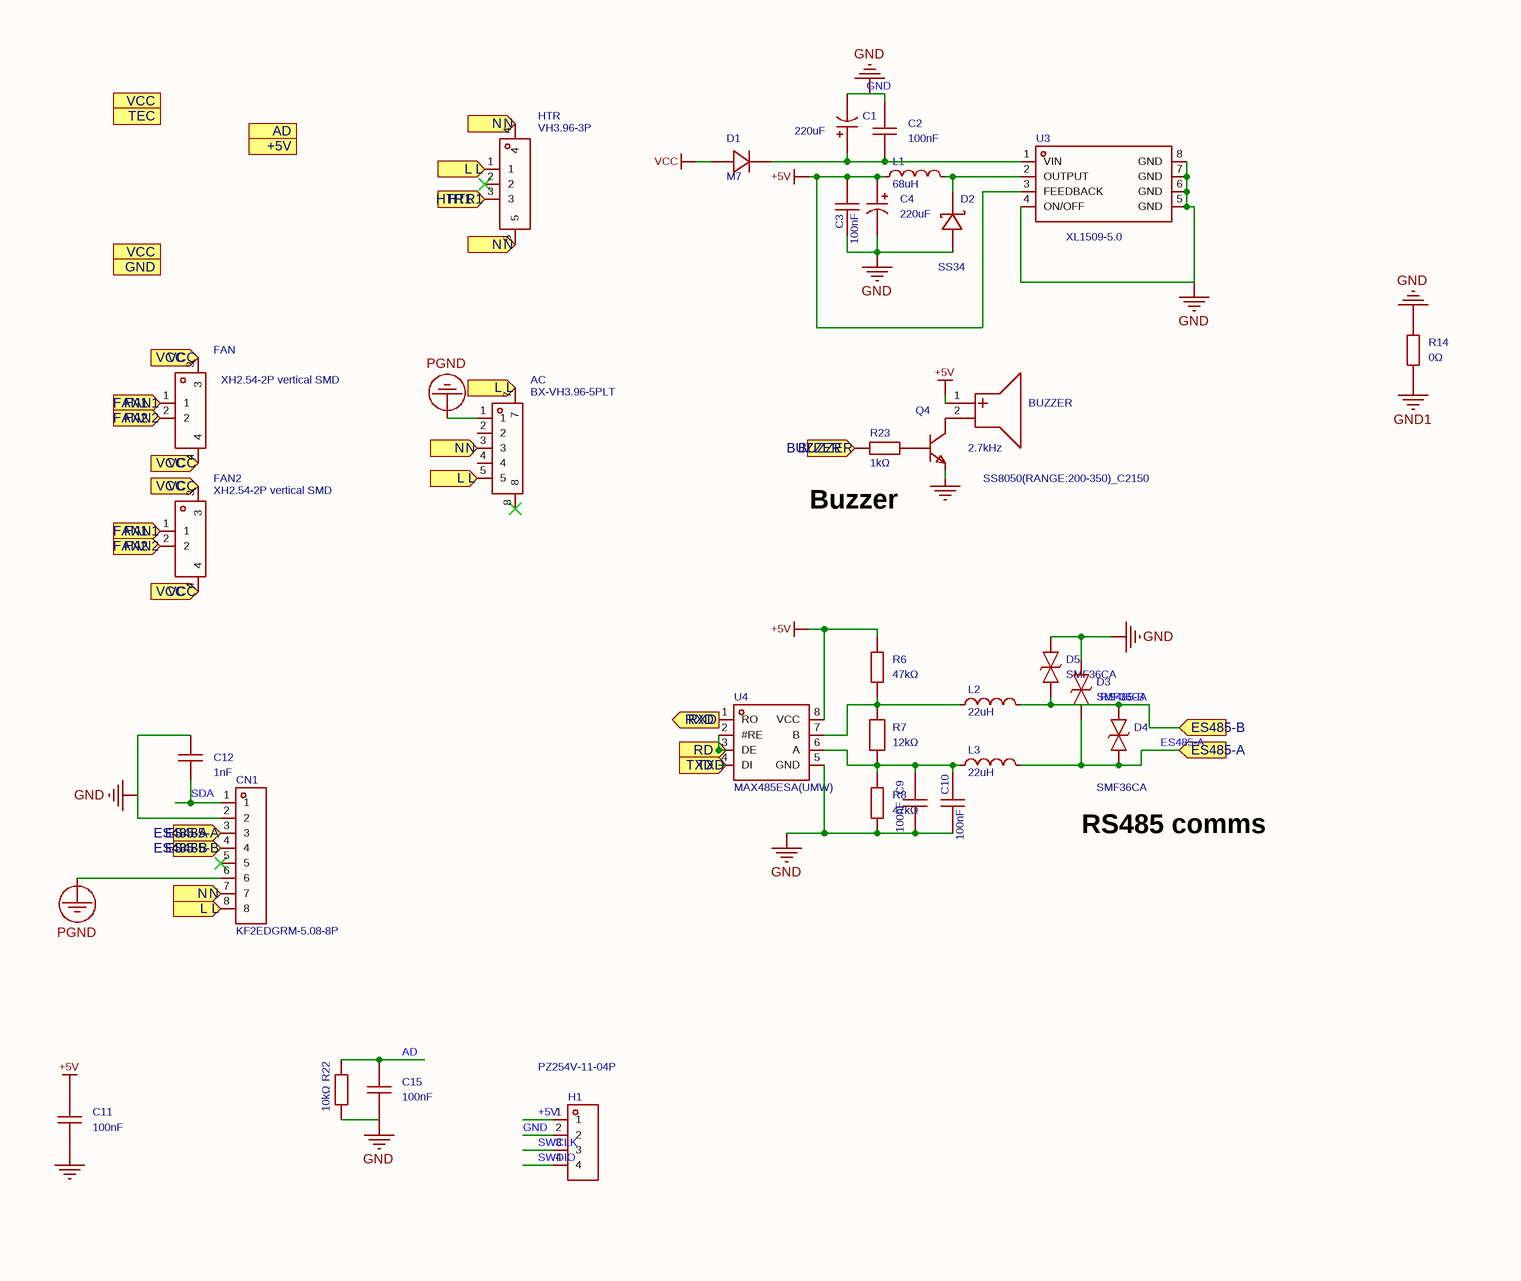
[diagram p0: MISC84275-2.SchDoc, left]
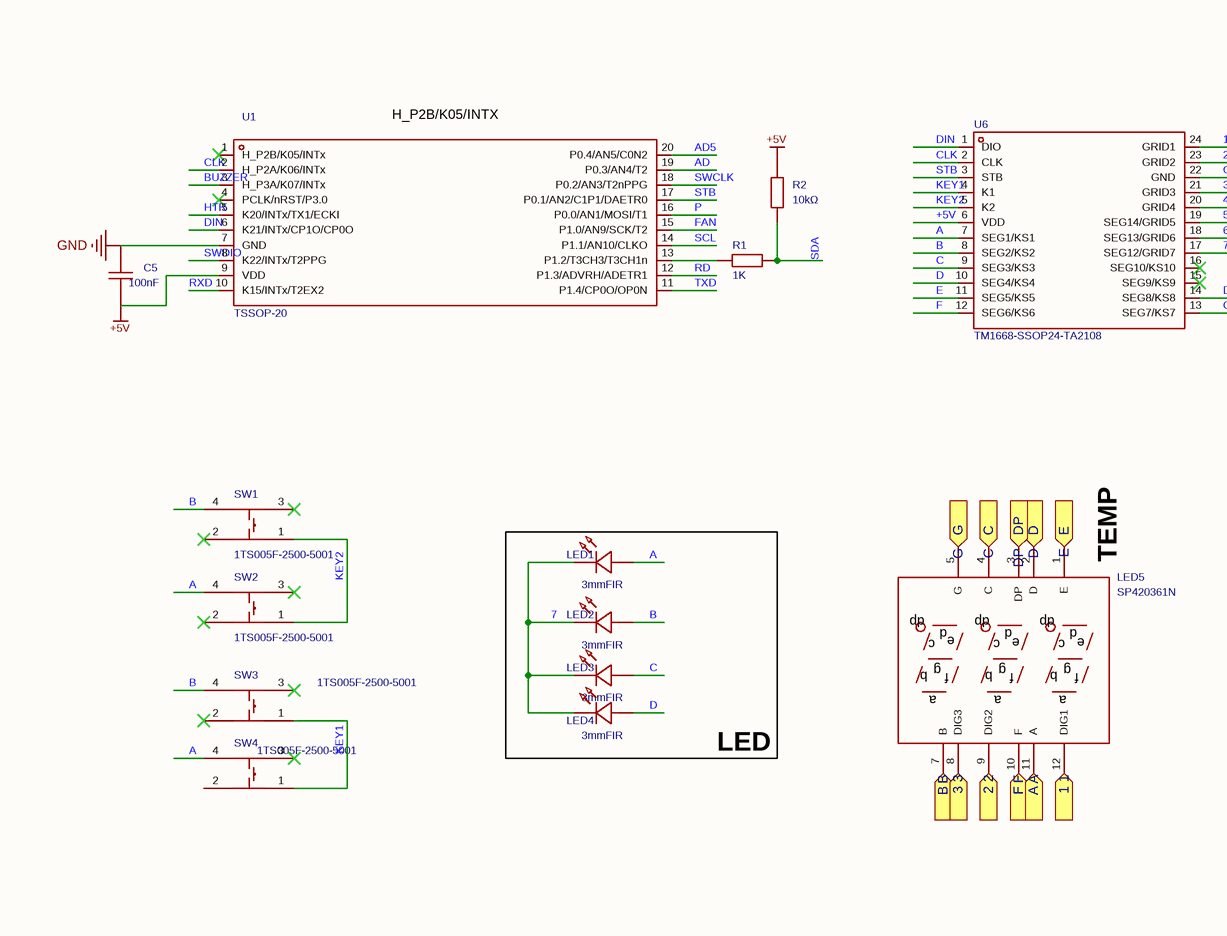
[diagram p1: MISC84275-2.SchDoc, middle]
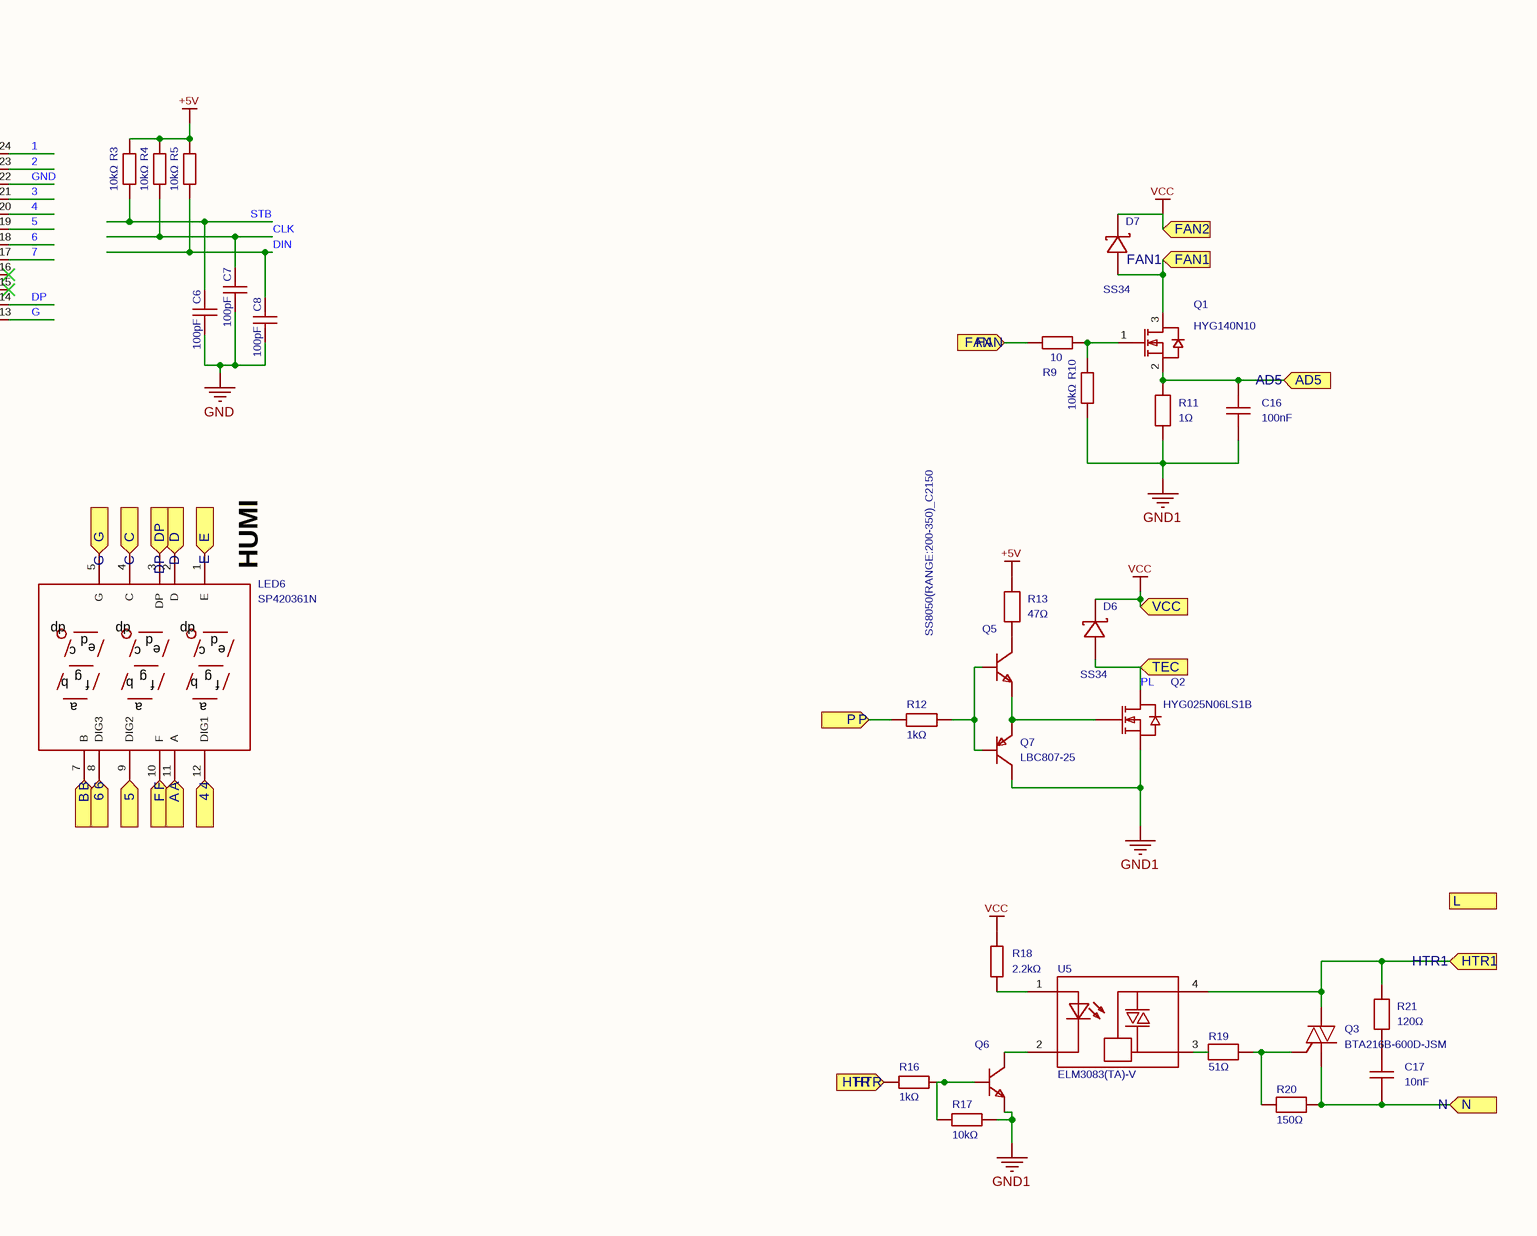
[diagram p2: MISC84275-2.SchDoc, right]
# Altium project MISC84275.PrjPcb (part 1 of 2)
1 sheet, 76 parts. Net scope: flat (ports and power ports of the same name join across sheets).
Board file: MISC84275.PcbDoc

## Sheet MISC84275-2.SchDoc
size 297 x 209 mm; Symbol: Drawing-Symbol_A4; Company: JLCEDA; Version: V1.0; Page Size: A4; @Project Name: Dehumidifier; @Page Count: 2; @Update Date: 2025-12-25; @Create Date: 2025-12-25; @Schematic Name: EDA-2150; @Page No: 1; @Page Name: P1; @Create Time: 08:36:43; @Update Time: 17:27:34; Border: 1; Width: 1170; Height: 825; Region Start: 1; X Region Count: 6; Y Region Count: 4; Blade Width: 10; Title Block Position: 3; @Board Name: EDA-2150; Device: Drawing-Symbol_A4

### Parts
AC  BX-VH3.96-5PLT  [CONN-SMD_5P-P3.96_BX-VH3.96-5PLT]
BUZZER  2.7kHz  [BUZ-SMD_L9.6-W9.6-LS10.0-R]
C1  220uF  [CAP-SMD_BD6.3-L6.6-W6.6-FD]
C2  100nF  [C0805]
C3  100nF  [C0805]
C4  220uF  [CAP-SMD_BD6.3-L6.6-W6.6-FD]
C5  100nF  [C0805]
C6  100pF  [C0805]
C7  100pF  [C0805]
C8  100pF  [C0805]
C9  100nF  [C0805]
C10  100nF  [C0805]
C11  100nF  [C0805]
C12  1nF  [C0805]
C15  100nF  [C0805]
C16  100nF  [C0805]
C17  10nF  [C1210]
CN1  KF2EDGRM-5.08-8P  [CONN-TH_8P-P5.08_KF2EDGRM-5.08-8P]
D1  M7  [SMA_L4.4-W2.8-LS5.4-RD]
D2  SS34  [SMA_L4.3-W2.6-LS5.2-RD]
D3  SMF36CA  [SOD-123_L2.7-W1.8-LS3.7-BI]
D4  SMF36CA  [SOD-123_L2.7-W1.8-LS3.7-BI]
D5  SMF36CA  [SOD-123_L2.7-W1.8-LS3.7-BI]
D6  SS34  [SMA_L4.3-W2.6-LS5.2-RD]
D7  SS34  [SMA_L4.3-W2.6-LS5.2-RD]
FAN  XH2.54-2P vertical SMD  [CONN-SMD_2P_A2501WV-S]
FAN2  XH2.54-2P vertical SMD  [CONN-SMD_2P_A2501WV-S]
H1  PZ254V-11-04P  [HDR-TH_4P-P2.54-V-M]
HTR  VH3.96-3P  [CONN-SMD_3P-P3.96_HCTL_HC-VH-3ALT]
L1  68uH  [IND-SMD_L7.1-W6.6_H5.0]
L2  22uH  [L1206]
L3  22uH  [L1206]
LED1  3mmFIR  [LED-TH_BD3.0-P2.54-FD]
LED2  3mmFIR  [LED-TH_BD3.0-P2.54-FD]
LED3  3mmFIR  [LED-TH_BD3.0-P2.54-FD]
LED4  3mmFIR  [LED-TH_BD3.0-P2.54-FD]
LED5  SP420361N  [LED-SEG-TH_SP420361N]
LED6  SP420361N  [LED-SEG-TH_SP420361N]
Q1  HYG140N10  [TO-252-3_L6.6-W6.1-P4.58-LS10.1-BR]
Q2  HYG025N06LS1B  [TO-263-2_L10.2-W8.7-P5.08-LS15.1-BR]
Q3  BTA216B-600D-JSM  [TO-263-3_L10.2-W9.2-P5.08-LS15.4-BR]
Q4  SS8050(RANGE:200-350)  [SOT-23-3_L2.9-W1.3-P1.90-LS2.4-BR]  (value not drawn)
Q5  SS8050(RANGE:200-350)  [SOT-23-3_L2.9-W1.3-P1.90-LS2.4-BR]  (value not drawn)
Q6  SS8050(RANGE:200-350)  [SOT-23-3_L2.9-W1.3-P1.90-LS2.4-BR]  (value not drawn)
Q7  LBC807-25  [SOT-23-3_L2.9-W1.6-P1.90-LS2.8-BR]
R1  1K  [R0805]
R2  10kΩ  [R0805]
R3  10kΩ  [R0805]
R4  10kΩ  [R0805]
R5  10kΩ  [R0805]
R6  47kΩ  [R0805]
R7  12kΩ  [R0805]
R8  47kΩ  [R0805]
R9  10  [R0805]
R10  10kΩ  [R0805]
R11  1Ω  [R1206]
R12  1kΩ  [R0805]
R13  47Ω  [R0805]
R14  0Ω  [R0603]
R16  1kΩ  [R0805]
R17  10kΩ  [R0805]
R18  2.2kΩ  [R0805]
R19  51Ω  [R0204]
R20  150Ω  [R0204]
R21  120Ω  [R0204]
R22  10kΩ  [R0805]
R23  1kΩ  [R0805]
SW1  1TS005F-2500-5001  [SW-SMD_4P-L6.0-W6.0-P4.50-LS9.0-H2.5]
SW2  1TS005F-2500-5001  [SW-SMD_4P-L6.0-W6.0-P4.50-LS9.0-H2.5]
SW3  1TS005F-2500-5001  [SW-SMD_4P-L6.0-W6.0-P4.50-LS9.0-H2.5]
SW4  1TS005F-2500-5001  [SW-SMD_4P-L6.0-W6.0-P4.50-LS9.0-H2.5]
U1  TSSOP-20  [TSSOP-20_L6.5-W4.4-P0.65-LS6.4-BL]
U3  XL1509-5.0  [SOIC-8_L4.9-W3.9-P1.27-LS6.0-TR]
U4  MAX485ESA(UMW)  [SOP-8_L5.0-W4.0-P1.27-LS6.0-BL]
U5  ELM3083(TA)-V  [SOP-4_L4.4-W4.0-P2.54-LS7.0-TL]
U6  TM1668-SSOP24-TA2108  [SSOP-24_L8.1-W5.3-P0.65-LS7.8-BL]

### Blocks framed on the sheet
LED: LED1-LED4

### Ports
1 (in), 2 (in), 3 (in), 4 (in), 5 (in), 6 (in), +5V (in), A (in), AD5 (in), AD (in), B (in), BUZZER (in), C (in), D (in), DP (in), E (in), ES485-A (in), ES485-B (in), F (in), FAN1 (in), FAN2 (in), FAN (in), G (in), GND (in), HTR1 (in), HTR (in), L (in), N (in), P (in), RD (in), RXD (out), TEC (in), TXD (in), VCC (in)

### Nets
+5V: BUZZER.1(+) C3.2 C4.1 C5.1 C11.2 H1.1 L1.1 R2.2 R3.2 R4.2 R5.2 R6.2 R13.2 U1.9(VDD) U3.3(FEEDBACK) U4.8(VCC) U6.6(VDD)
VCC: D1.2(A) D6.1(K) D7.1(K) FAN.2 FAN.3 FAN.4 FAN2.2 FAN2.3 FAN2.4 R18.2 ; port VCC, port FAN2  [also labelled FAN2]
GND: C1.2 C2.2 C3.1 C4.2 C5.2 C6.1 C7.1 C8.1 C9.1 C10.1 C11.1 C12.2 C15.1 CN1.2 D2.2(A) D3.2 D5.2 H1.2 Q4.2(E) R8.1 R14.2 R22.1 U1.7(GND) U3.4(ON/OFF) U3.5(GND) U3.6(GND) U3.7(GND) U3.8(GND) U4.5(GND) U6.22(GND)
GND1: C16.1 Q2.3(S) Q6.2(E) Q7.3 R10.1 R11.1 R14.1 R17.2
PGND: AC.1 CN1.6
1: LED5.12(DIG1) U6.24(GRID1) ; port 1
2: LED5.9(DIG2) U6.23(GRID2) ; port 2
3: LED5.8(DIG3) U6.21(GRID3) ; port 3
4: LED6.12(DIG1) U6.20(GRID4) ; port 4
5: U6.19(SEG14/GRID5)
6: LED6.8(DIG3) U6.18(SEG13/GRID6) ; port 6
7: LED1.2(K) LED2.2(K) LED3.2(K) LED4.2(K) U6.17(SEG12/GRID7)
A: LED1.1(A) LED5.11(A) LED6.11(A) SW2.4 SW4.4 U6.7(SEG1/KS1) ; port A
AD: C15.2 R22.2 U1.19(P0.3/AN4/T2)
AD5: C16.2 Q1.2(S) R11.2 U1.20(P0.4/AN5/C0N2) ; port AD5
B: LED2.1(A) LED5.7(B) LED6.7(B) SW1.4 SW3.4 U6.8(SEG2/KS2) ; port B
BUZZER: R23.1 U1.3(H_P3A/K07/INTx) ; port BUZZER
C: LED3.1(A) LED5.4(C) LED6.4(C) U6.9(SEG3/KS3) ; port C
CLK: C7.2 R4.1 U1.2(H_P2A/K06/INTx) U6.2(CLK)
D: LED4.1(A) LED5.2(D) LED6.2(D) U6.10(SEG4/KS4) ; port D
DIN: C8.2 R5.1 U1.6(K21/INTx/CP1O/CP0O) U6.1(DIO)
DP: LED5.3(DP) LED6.3(DP) U6.14(SEG8/KS8) ; port DP
E: LED5.1(E) LED6.1(E) U6.11(SEG5/KS5) ; port E
ES485-A: CN1.3 D3.1 D4.1 L3.2 ; port ES485-A
ES485-B: CN1.4 D4.2 D5.1 L2.2 ; port ES485-B  [also labelled RS485-B]
F: LED5.10(F) LED6.10(F) U6.12(SEG6/KS6) ; port F
FAN: R9.1 U1.15(P1.0/AN9/SCK/T2) ; port FAN
FAN1: D7.2(A) FAN.1 FAN2.1 Q1.3(D) ; port FAN1
G: LED5.5(G) LED6.5(G) U6.13(SEG7/KS7) ; port G
HTR: R16.1 U1.5(K20/INTx/TX1/ECKI) ; port HTR
HTR1: HTR.3 Q3.2(T2) R21.2 U5.4(Terminal) ; port HTR1
KEY1: SW3.1 SW4.1 U6.4(K1)
KEY2: SW1.1 SW2.1 U6.5(K2)
L: AC.5 AC.7 CN1.8 HTR.1 ; port L
N: AC.3 C17.1 CN1.7 HTR.4 HTR.5 Q3.1(T1) R20.2 ; port N
P: R12.1 U1.16(P0.0/AN1/MOSI/T1) ; port P
PL: D6.2(A) Q2.4(D) ; port TEC
RD: U1.12(P1.3/ADVRH/ADETR1)
RXD: U1.10(K15/INTx/T2EX2) U4.1(RO) ; port RXD
SCL: U1.14(P1.1/AN10/CLKO)
SDA: C12.1 CN1.1 R1.2 R2.1
STB: C6.2 R3.1 U1.17(P0.1/AN2/C1P1/DAETR0) U6.3(STB)
SWCLK: H1.3 U1.18(P0.2/AN3/T2nPPG)
SWDIO: H1.4 U1.8(K22/INTx/T2PPG)
TXD: U1.11(P1.4/CP0O/OP0N) U4.4(DI) ; port TXD
NetBUZZER_2: BUZZER.2(-) Q4.3(C)
NetC1_1: C1.1 C2.1 D1.1(K) U3.1(VIN)
NetC9_2: C9.2 C10.2 L3.1 R7.1 R8.2 U4.6(A)
NetC17_2: C17.2 R21.1
NetD2_1: D2.1(K) L1.2 U3.2(OUTPUT)
NetL2_1: L2.1 R6.1 R7.2 U4.7(B)
NetLED6_9: LED6.9(DIG2) ; port 5
NetQ1_1: Q1.1(G) R9.2 R10.2
NetQ2_1: Q2.1(G) Q5.2(E) Q7.2
NetQ3_3: Q3.3(G) R19.2 R20.1
NetQ4_1: Q4.1(B) R23.2
NetQ5_1: Q5.1(B) Q7.1 R12.2
NetQ5_3: Q5.3(C) R13.1
NetQ6_1: Q6.1(B) R16.2 R17.1
NetQ6_3: Q6.3(C) U5.2(Cathode)
NetR1_1: R1.1 U1.13(P1.2/T3CH3/T3CH1n)
NetR18_1: R18.1 U5.1(ANODE)
NetR19_1: R19.1 U5.3(Terminal)
NetU4_2: U4.2(#RE) U4.3(DE) ; port RD

Not connected (* = marked no-connect by the designer): AC 2 4 8*; CN1 5*; HTR 2*; SW1 2* 3*; SW2 2* 3*; SW3 2* 3*; SW4 2 3*; U1 1(H_P2B/K05/INTx)* 4(PCLK/nRST/P3.0)*; U6 15(SEG9/KS9)* 16(SEG10/KS10)*

### Notes on the sheet
- Buzzer
- (near LED5) TEMP
- (near LED6) HUMI
- RS485 comms
- Created
- 2025-12-25
- Schematic
- Board
- EDA-2150
- Updated
- Sheet
- P1
- Drawn
- Reviewed
- Dehumidifier
- Revision
- V1.0
- Size
- A4
- Sheet    1    of    2
- JLCEDA

### Library data of the parts
AC = BX-VH3.96-5PLT: Pin structure:1x5P;Pitch:3.96mm;Mounting:Vertical SMD;Series:VH;Total pins:5P;Rows:1;Pins per row:5;Row spacing:-;Rated current:7A;Contact material:Brass;Contact plating:Tin;Operating temp:-25℃~+85℃;; Manufacturer: Bossie(博锡); AddInBom: yes; ModelId: 3eef25eeae864211af0ae444696b206f0819f05c4eef4c71ace90d822a990e87; ModelTransform: 935.4312,484.255,0,180,0,0,0,0,0; Pins Structure: 1x5P; Pitch: 3.96mm; Reference Series: VH; Number of PINs Per Row: 5; Current Rating: 7A; Voltage Rating: 250V; Plastic Material: LCP; Flame Retardant Rating: UL94V-0; Supplementary Features: Auxiliary solder tabs; Z-Height of the Board: 11.6mm; X-Length of Bottom Edge on Board (Spacing Line): 23.76mm; Symbol: BX-VH3.96-5PLT; Device: BX-VH3.96-5PLT; LCSC Part Name: 1x5P 间距:3.96mm 立贴 系列:VH; SupplierPart: C18077854; ManufacturerPart: BX-VH3.96-5PLT; Supplier Footprint: SMD,P=3.96mm; JLCPCB Part Class: Extended Part; Datasheet: https://item.szlcsc.com/datasheet/BX-VH3.96-5PLT/19218255.html; Supplier: LCSC; ConvertToPcb: yes; FootprintName: CONN-SMD_5P-P3.96_BX-VH3.96-5PLT; ModelName: CONN-SMD_5P-P3.96_BX-VH3.96-5PLT; Mounting Type: Vertical SMD; Number of Pins: 5P; Number of Rows: 1; Row Spacing: -; Contact Material: Brass; Contact Plating: Tin; Operating Temperature: -25℃~+85℃; Color: Beige; Y-Width of Bottom Edge on Board: -
BUZZER = YS-SBZ9650DYB05: Drive:Active(built-in driver circuit);Frequency:2.7kHz;Sound pressure(SPL):80dB;; Manufacturer: Fengming(锋鸣电子); Symbol: YS-SBZ9650DYB05_C409830; 3D Model: d9f071f9511e4f7795b1f85db8085480; 3D Model Transform: 393.7,377.952,0,0,0,0,0,0,0; Voltage - Supply: 3V~7V; Sound Pressure Level(SPL): 80dB; AddInBom: yes; ModelName: BUZ-SMD_L9.6-W9.6-H5.0; Device: YS-SBZ9650DYB05; LCSC Part Name: 贴片有源蜂鸣器5V; Supplier Part: C409830; Manufacturer Part: YS-SBZ9650DYB05; Supplier Footprint: SMD,9.6x9.6mm; JLCPCB Part Class: Extended library; Datasheet: https://item.szlcsc.com/datasheet/YS-SBZ9650DYB05/400193.html; Supplier: LCSC; Driver Circuitry: Active(built-in driver circuit); Value: 2.7kHz; Length: 9.6mm; Width: 9.6mm; Height: 5.3mm; ConvertToPcb: yes; FootprintName: BUZ-SMD_L9.6-W9.6-LS10.0-R
C1 C4 = JVJ35V220M6x8: Capacitance:220uF;Tolerance:±20%;Rated voltage:35V;Ripple current:190mA@120Hz;; Manufacturer: JIERR(捷而瑞); AddInBom: yes; ModelId: ec7f1c7bda5e4386b54ec5ff3d1d94ff; ModelTransform: 307.086,259.842,0,180,0,0,0,0,0; Tolerance: ±20%; Voltage Rating: 35V; Lifetime: 2000hrs@105℃; Symbol: JVJ35V220M6X8; Device: JVJ35V220M6x8; LCSC Part Name: 220uF ±20% 35V; SupplierPart: C46550411; ManufacturerPart: JVJ35V220M6x8; Supplier Footprint: SMD,D6.3xL7.7mm; JLCPCB Part Class: Extended library; Datasheet: https://item.szlcsc.com/datasheet/JVJ35V220M6x8/48680105.html; Supplier: LCSC; ConvertToPcb: yes; FootprintName: CAP-SMD_BD6.3-L6.6-W6.6-FD; ModelName: CAP-SMD_BD6.3-L6.6-W6.6-FD; Value: 220uF; Ripple Current: 190mA@120Hz; Diameter: 6.3mm; Height - Seated (Max): 7.7mm; Operating Temperature: -55℃~+105℃
C2 C3 C11 = FCC0805B104K500DT: Capacitance:100nF;Tolerance:±10%;Rated voltage:50V;Temp coefficient:X7R;; Manufacturer: FOJAN(富捷); AddInBom: yes; ModelId: 1ba041120af144c991958decab20d2410819f05c4eef4c71ace90d822a990e87; ModelName: C0805_L2.0-W1.3-H1.3; ModelTransform: 78.74,51.181,0,0,0,0,0,0.0005,0; Tolerance: ±10%; Voltage Rating: 50V; Temperature Coefficient: X7R; Symbol: FCC0805B104K500DT; Device: FCC0805B104K500DT; LCSC Part Name: 100nF ±10% 50V; SupplierPart: C5137467; ManufacturerPart: FCC0805B104K500DT; Supplier Footprint: 0805; JLCPCB Part Class: Extended Part; Datasheet: https://item.szlcsc.com/datasheet/FCC0805B104K500DT/5746969.html; Supplier: LCSC; ConvertToPcb: yes; FootprintName: C0805; Value: 100nF
C5 C9 C10 C15 C16 = FCC0805B104K500DT: Capacitance:100nF;Tolerance:±10%;Rated voltage:50V;Temp coefficient:X7R;; Manufacturer: FOJAN(富捷); 3D Model: 1ba041120af144c991958decab20d2410819f05c4eef4c71ace90d822a990e87; 3D Model Transform: 78.74,51.181,0,0,0,0,0,0.0005,0; Tolerance: ±10%; Voltage Rating: 50V; Temperature Coefficient: X7R; AddInBom: yes; ModelName: C0805_L2.0-W1.3-H1.3; Symbol: FCC0805B104K500DT; Device: FCC0805B104K500DT; LCSC Part Name: 100nF ±10% 50V; Supplier Part: C5137467; Manufacturer Part: FCC0805B104K500DT; Supplier Footprint: 0805; JLCPCB Part Class: Extended Part; Datasheet: https://item.szlcsc.com/datasheet/FCC0805B104K500DT/5746969.html; Supplier: LCSC; Value: 100nF; ConvertToPcb: yes; FootprintName: C0805
C6-C8 = CL21C101JBANNNC: Capacitance:100pF;Tolerance:±5%;Rated voltage:50V;Temp coefficient:C0G;; Manufacturer: SAMSUNG(三星); 3D Model: 1ba041120af144c991958decab20d2410819f05c4eef4c71ace90d822a990e87; 3D Model Transform: 78.74,51.181,0,0,0,0,0,0.0005,0; Tolerance: ±5%; Voltage Rating: 50V; Temperature Coefficient: C0G; AddInBom: yes; ModelName: C0805_L2.0-W1.3-H1.3; Symbol: CL21C101JBANNNC; Device: CL21C101JBANNNC; LCSC Part Name: 100pF ±5% 50V; Supplier Part: C1790; Manufacturer Part: CL21C101JBANNNC; Supplier Footprint: 0805; JLCPCB Part Class: Basic Part; Datasheet: https://item.szlcsc.com/datasheet/CL21C101JBANNNC/2142.html; Supplier: LCSC; Value: 100pF; ConvertToPcb: yes; FootprintName: C0805
C12 = CL21B102KBCNNNC: Capacitance:1nF;Tolerance:±10%;Rated voltage:50V;Temp coefficient:X7R;; Manufacturer: SAMSUNG(三星); AddInBom: yes; ModelId: 1ba041120af144c991958decab20d2410819f05c4eef4c71ace90d822a990e87; ModelName: C0805_L2.0-W1.3-H1.3; ModelTransform: 78.74,51.181,0,0,0,0,0,0.0005,0; Tolerance: ±10%; Voltage Rating: 50V; Temperature Coefficient: X7R; Symbol: CL21B102KBCNNNC; Device: CL21B102KBCNNNC; LCSC Part Name: 1nF ±10% 50V; SupplierPart: C46653; ManufacturerPart: CL21B102KBCNNNC; Supplier Footprint: 0805; JLCPCB Part Class: Basic Part; Datasheet: https://item.szlcsc.com/datasheet/CL21B102KBCNNNC/47657.html; Supplier: LCSC; ConvertToPcb: yes; FootprintName: C0805; Value: 1nF
C17 = 1210B103K500NT: Capacitance:10nF;Tolerance:±10%;Rated voltage:50V;Temp coefficient:X7R;; Manufacturer: FH(风华); 3D Model: 833068e7fe044595a6eec77c56179455; 3D Model Transform: 125.984,98.425,0,0,0,0,0,0,0; Tolerance: ±10%; Voltage Rating: 50V; Temperature Coefficient: X7R; AddInBom: yes; ModelName: C1210_L3.2-W2.5-H2.5; Symbol: 1210B103K500NT; Device: 1210B103K500NT; LCSC Part Name: 10nF ±10% 50V; Supplier Part: C20616768; Manufacturer Part: 1210B103K500NT; Supplier Footprint: 1210; JLCPCB Part Class: Extended library; Datasheet: https://item.szlcsc.com/datasheet/1210B103K500NT/21984757.html; Supplier: LCSC; Value: 10nF; ConvertToPcb: yes; FootprintName: C1210
CN1 = KF2EDGRM-5.08-8P: Connector type:Board-side socket, closed;Fixing:Screw;Structure:1x8P;Pitch:5.08mm;Colour:Green;Mounting:Right-angle THT;Rows:1;Pins per row:8;Rated current:15A;Rated voltage:300V;Operating temp:-40℃~+105℃;; Manufacturer: KEFA(科发); AddInBom: yes; ModelId: 46f925dc5c95482eafe175578533ed310819f05c4eef4c71ace90d822a990e87; ModelTransform: 2001.5708,488.188,0,0,0,0,0,-192.913,-165.354; Number of Positions or Pins: 1x8P; Pitch: 5.08mm; Number of PINs Per Row: 8; Current Rating: 15A; Voltage Rating (Max): 300V; Symbol: KF2EDGRM-5.08-8P; Device: KF2EDGRM-5.08-8P; LCSC Part Name: 螺丝固定 1x8P 5.08mm 排数:1 每排P数:8; SupplierPart: C441294; ManufacturerPart: KF2EDGRM-5.08-8P; Supplier Footprint: 弯插,P=5.08mm; JLCPCB Part Class: Extended Part; Datasheet: https://item.szlcsc.com/datasheet/KF2EDGRM-5.08-8P/441267.html; Supplier: LCSC; ConvertToPcb: yes; FootprintName: CONN-TH_8P-P5.08_KF2EDGRM-5.08-8P; ModelName: CONN-TH_8P-P5.08_KF2EDGRM-5.08-8P; Connector Type: Board-side socket, closed; Termination Style: Screw; Color: Green; Mounting Type: Right-angle THT; Number of Pins: 8P; Number of Rows: 1; Operating Temperature: -40℃~+105℃
D1 = M7_C46598121: Diode configuration:1 single;Forward voltage(Vf):1.1V@1A;DC reverse voltage(Vr):1kV;Rectified current:1A;; Manufacturer: baocheng(宝乘); AddInBom: yes; ModelId: 4f1e9ef2303f48b48aa8ce0cacf8d7b10819f05c4eef4c71ace90d822a990e87; ModelTransform: 204.724,102.362,0,0,0,0,0,0,0; Voltage - DC Reverse(Vr): 1kV; Current - Rectified: 1A; Reverse Leakage Current (Ir): 5uA; Non-Repetitive Peak Forward Surge Current: 30A; Operating Junction Temperature Range: -55℃~+150℃; Symbol: M7_C46598121; Device: M7_C46598121; LCSC Part Name: 贴片二极管; SupplierPart: C46598121; ManufacturerPart: M7; Supplier Footprint: SMA; Datasheet: https://item.szlcsc.com/datasheet/M7/48740327.html; Supplier: LCSC; ConvertToPcb: yes; FootprintName: SMA_L4.4-W2.8-LS5.4-RD; ModelName: SMA_L4.4-W2.8-LS5.4-RD; Diode Configuration: 1 single; Voltage - Forward(Vf@If): 1.1V@1A